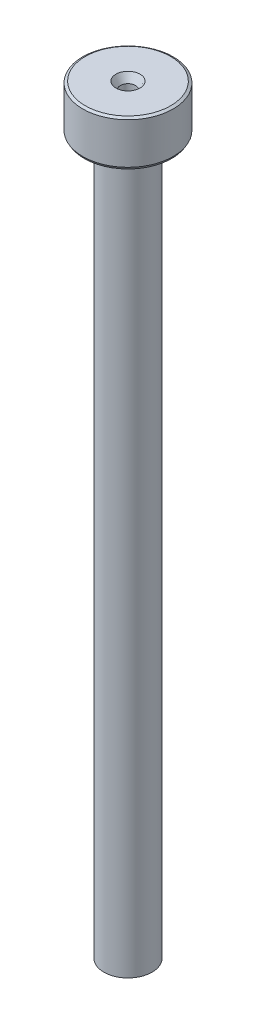
from build123d import *
from OCP.BRepFilletAPI import BRepFilletAPI_MakeChamfer

# Parameters (mm, degrees)
F_5_0MM_DOWEL_HOLE1_D     = 5
F_5_0MM_DOWEL_HOLE1_DEPTH = 5
F_5_0MM_DOWEL_HOLE1_TIP   = 1.502151548
CHAMFER1_SIZE             = 1.5
CHAMFER1_SIZE2            = 2.496419224
CHAMFER2_SIZE             = 0.5
CHAMFER2_SIZE2            = 0.832139741
F_5_0MM_DOWEL_HOLE2_D     = 5
F_5_0MM_DOWEL_HOLE2_DEPTH = 5
F_5_0MM_DOWEL_HOLE2_TIP   = 1.502151548
CHAMFER3_SIZE             = 1.5
CHAMFER3_SIZE2            = 2.496419224


with BuildPart() as part:
    # Sketch1 → Revolve1 (revolve)
    with BuildSketch(Plane.XY, mode=Mode.PRIVATE) as revolve1_sk:
        Polygon((0, 252), (15, 252), (15, 237), (6, 237), (6, 233), (8, 233), (8, 0), (0, 0), align=None)
    revolve(revolve1_sk.sketch.rotate(Axis((0, 252, 0), (0, -1, 0)), 180), axis=Axis((0, 252, 0), (0, -1, 0)))

    # Ø5.0mm Dowel Hole1
    with Locations(Plane(origin=(0, 0, 0), x_dir=(-1, 0, 0), z_dir=(0, -1, 0))):
        with Locations((0, 0), (163.193456079, -92.802944279)):
            Hole(F_5_0MM_DOWEL_HOLE1_D / 2, depth=F_5_0MM_DOWEL_HOLE1_DEPTH)
            with Locations((0, 0, -(F_5_0MM_DOWEL_HOLE1_DEPTH + F_5_0MM_DOWEL_HOLE1_TIP / 2))):  # 118° drill point
                Cone(0, F_5_0MM_DOWEL_HOLE1_D / 2, F_5_0MM_DOWEL_HOLE1_TIP, mode=Mode.SUBTRACT)

    # Chamfer1
    chamfer1_edges = [part.edges().sort_by_distance(p)[0] for p in [
        (-2.5, 0, 0),
    ]]
    chamfer1_side = [part.faces().sort_by_distance(p)[0] for p in [
        (7.77372583, 0, 0),
    ]]
    chamfer(chamfer1_edges, length=CHAMFER1_SIZE, length2=CHAMFER1_SIZE2, reference=chamfer1_side[0])

    # Chamfer2: one chamfer whose edges measure the first distance from different faces: ONE call of the kernel's chamfer builder (chamfer() names one face for all edges)
    chamfer2_edges_1 = [part.edges().sort_by_distance(p)[0] for p in [
        (15, 237, 0),
    ]]
    chamfer2_side_1 = [part.faces().sort_by_distance(p)[0] for p in [
        (14.575735931, 237, 0),
    ]]
    chamfer2_edges_2 = [part.edges().sort_by_distance(p)[0] for p in [
        (15, 252, 0),
    ]]
    chamfer2_side_2 = [part.faces().sort_by_distance(p)[0] for p in [
        (15, 244.5, 0),
    ]]
    chamfer2_edges_3 = [part.edges().sort_by_distance(p)[0] for p in [
        (8, 233, 0),
    ]]
    chamfer2_side_3 = [part.faces().sort_by_distance(p)[0] for p in [
        (8, 116.5, 0),
    ]]
    chamfer2 = BRepFilletAPI_MakeChamfer(part.part.solid().wrapped)
    for e in chamfer2_edges_1:
        chamfer2.Add(CHAMFER2_SIZE, CHAMFER2_SIZE2, e.wrapped, chamfer2_side_1[0].wrapped)  # the first distance lies on this face
    for e in chamfer2_edges_2:
        chamfer2.Add(CHAMFER2_SIZE, CHAMFER2_SIZE2, e.wrapped, chamfer2_side_2[0].wrapped)  # the first distance lies on this face
    for e in chamfer2_edges_3:
        chamfer2.Add(CHAMFER2_SIZE, CHAMFER2_SIZE2, e.wrapped, chamfer2_side_3[0].wrapped)  # the first distance lies on this face
    add(Compound.cast(chamfer2.Shape()), mode=Mode.REPLACE)

    # Ø5.0mm Dowel Hole2
    with Locations(Plane(origin=(0, 252, 0), x_dir=(1, 0, 0), z_dir=(0, 1, 0))):
        with Locations((0, 0)):
            Hole(F_5_0MM_DOWEL_HOLE2_D / 2, depth=F_5_0MM_DOWEL_HOLE2_DEPTH)
            with Locations((0, 0, -(F_5_0MM_DOWEL_HOLE2_DEPTH + F_5_0MM_DOWEL_HOLE2_TIP / 2))):  # 118° drill point
                Cone(0, F_5_0MM_DOWEL_HOLE2_D / 2, F_5_0MM_DOWEL_HOLE2_TIP, mode=Mode.SUBTRACT)

    # Chamfer3
    chamfer3_edges = [part.edges().sort_by_distance(p)[0] for p in [
        (2.5, 252, 0),
    ]]
    chamfer3_side = [part.faces().sort_by_distance(p)[0] for p in [
        (13.767132656, 252, 0),
    ]]
    chamfer(chamfer3_edges, length=CHAMFER3_SIZE, length2=CHAMFER3_SIZE2, reference=chamfer3_side[0])


solid = part.part
